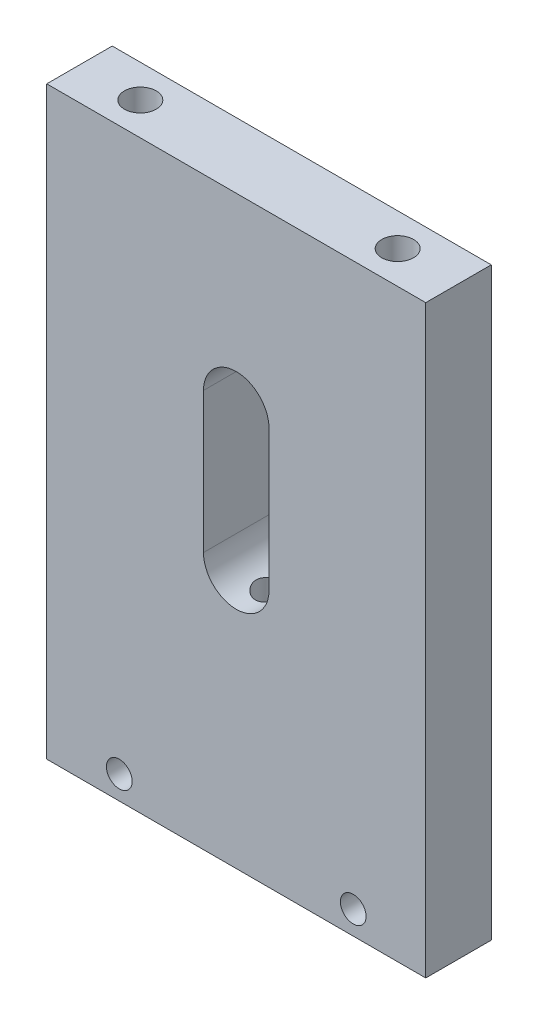
SolidWorks part; units mm, degrees
ref_plane "前视" through (0, 0, 0) normal (0, 0, 1) x (1, 0, 0)
ref_plane "上视" through (0, 0, 0) normal (0, 1, 0) x (1, 0, 0)
ref_plane "右视" through (0, 0, 0) normal (1, 0, 0) x (0, 0, -1)
sketch "草图1" plane through (0, 0, 0) normal (0, 0, 1) x (1, 0, 0)
  line L1 (0, 0) -> (81, 0)
  line L2 (0, 0) -> (0, -125)
  line L3 (0, -125) -> (81, -125)
  line L4 (81, 0) -> (81, -125)
  dimension "D1" = 81
  dimension "D2" = 125
extrude "凸台-拉伸1" add sketch "草图1" along normal blind 14
sketch "草图2" plane through (0, 0, 14) normal (0, 0, 1) x (1, 0, 0)
  line L0 (40.5, -55) -> (40.5, -125) construction
  line L1 (0, -125) -> (81, -125) construction
  line L2 (40.5, -70) -> (40.5, -40) construction
  line L3 (33.5, -70) -> (33.5, -40)
  line L4 (47.5, -70) -> (47.5, -40)
  arc A0 (33.5, -70) -> (47.5, -70) centre (40.5, -70) ccw
  arc A1 (47.5, -40) -> (33.5, -40) centre (40.5, -40) ccw
  point P6 (40.5, -55)
  dimension "D1" = 14
  dimension "D2" = 70
  dimension "D3" = 30
extrude "切除-拉伸1" cut sketch "草图2" against normal through all
sketch "草图4" plane through (70, -125, 0) normal (0, -1, 0) x (0, 0, -1)
  line L0 (-7, -29) -> (-7, 11) construction
  line L2 (-14, 11) -> (0, 11) construction
  circle A0 centre (-7, -29) radius 3.25
  dimension "D2" = 6.5
  dimension "D1" = 40
extrude "切除-拉伸2" cut sketch "草图4" against normal up to surface (48.0179 mm away)
cosmetic thread "装饰螺纹线1" parameters "D2"=8
cosmetic thread "装饰螺纹线2" parameters "D2"=8
hole_wizard "M8 螺纹孔1" positions "草图6" profile "草图5" tap size "M8" standard "GB"
sketch "草图6" plane through (0, 0, 0) normal (0, 1, 0) x (1, 0, 0)
  line L0 (40.5, -14) -> (40.5, 7.1905) construction
  line L1 (81, -14) -> (0, -14) construction
  line L3 (0, -7) -> (24.2024, -7) construction
  line L4 (0, -14) -> (0, 0) construction
  point P0 (68, -7)
  point P3 (13, -7)
  dimension "D1" = 55
sketch "草图5" plane through (68, 0, 7) normal (1, 0, 0) x (0, 0, 1)
  line L0 (0, 0) -> (0, 24.2929)
  line L1 (0, 24.2929) -> (3.4, 22.25)
  line L2 (3.4, 22.25) -> (3.4, 0)
  line L5 (3.4, 0) -> (0, 0)
  line L10 (0, 24.2929) -> (-3.4, 22.25) construction
  line L11 (0, -6.35) -> (0, 107.95) construction
  dimension "螺纹孔钻头直径" = 6.8
  dimension "螺纹孔钻头深度" = 22.25
  dimension "导头角度" = 118
cosmetic thread "孔螺蚊线1" parameters "D1"=16, "D2"=8
cosmetic thread "孔螺蚊线2" parameters "D1"=16, "D2"=8
sketch "草图11" plane through (0, 0, 14) normal (0, 0, 1) x (1, 0, 0)
  line L0 (15.5, -120) -> (65.5, -120) construction
  line L1 (40.5, -120) -> (40.5, -125) construction
  line L2 (0, -125) -> (81, -125) construction
  circle A0 centre (15.5, -120) radius 2.75
  circle A1 centre (65.5, -120) radius 2.75
  dimension "D3" = 5.5
  dimension "D1" = 50
  dimension "D2" = 5
extrude "切除-拉伸3" cut sketch "草图11" against normal through all
